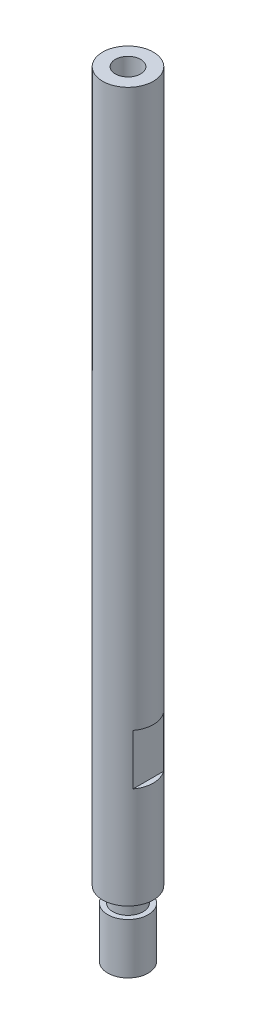
SolidWorks part; units mm, degrees
ref_plane "Front Plane" through (0, 0, 0) normal (0, 0, 1) x (1, 0, 0)
ref_plane "Top Plane" through (0, 0, 0) normal (0, 1, 0) x (1, 0, 0)
ref_plane "Right Plane" through (0, 0, 0) normal (1, 0, 0) x (0, 0, -1)
sketch "Sketch1" plane through (0, 0, 0) normal (0, 0, 1) x (1, 0, 0)
  line L0 (0, 14.171) -> (0, -138.829)
  line L1 (0, -138.829) -> (-4, -138.829)
  line L2 (-4, -138.829) -> (-4, -128.829)
  line L3 (-4, -128.829) -> (-3, -128.829)
  line L4 (-3, -128.829) -> (-3, -125.829)
  line L5 (-3, -125.829) -> (-5, -125.829)
  line L6 (-5, -125.829) -> (-5, 14.171)
  line L7 (-5, 14.171) -> (0, 14.171)
  dimension "D1" = 5
  dimension "D2" = 140
  dimension "D3" = 3
  dimension "D4" = 153
  dimension "D5" = 4
  dimension "D6" = 3
revolve "Revolve1" add sketch "Sketch1" angle 360 about L0
cosmetic thread "Cosmetic Thread1" parameters "D2"=6.647
sketch "Sketch2" plane through (0, 0, 0) normal (0, 0, 1) x (1, 0, 0)
  line L0 (-5, 14.171) -> (-5, -125.829) construction
  line L1 (-5, -95.829) -> (-4, -95.829)
  line L2 (-5, -95.829) -> (-5, -105.829)
  line L3 (-5, -105.829) -> (-4, -105.829)
  line L4 (-4, -95.829) -> (-4, -105.829)
  line L5 (5, 14.171) -> (-5, 14.171) construction
  line L6 (0, -125.829) -> (0, -35.6063) construction
  line L7 (-3, -125.829) -> (3, -125.829) construction
  line L8 (4, -95.829) -> (4, -105.829)
  line L9 (5, -105.829) -> (4, -105.829)
  line L10 (5, -95.829) -> (5, -105.829)
  line L11 (5, -95.829) -> (4, -95.829)
  point P6 (-4.5, -95.829)
  dimension "D1" = 1
  dimension "D2" = 10
  dimension "D3" = 110
extrude "Cut-Extrude1" cut sketch "Sketch2" against normal through all both and the other way through all
hole_wizard "M6 Tapped Hole1" positions "Sketch3" profile "Sketch4" tap size "M6" standard "GB"
sketch "Sketch3" plane through (0, 14.171, 0) normal (0, 1, 0) x (1, 0, 0)
  point P0 (0, 0)
sketch "Sketch4" plane through (0, 14.171, 0) normal (1, 0, 0) x (0, 0, 1)
  line L0 (0, 0) -> (0, 13.5022)
  line L1 (0, 13.5022) -> (2.5, 12)
  line L2 (2.5, 12) -> (2.5, 0)
  line L5 (2.5, 0) -> (0, 0)
  line L10 (0, 13.5022) -> (-2.5, 12) construction
  line L11 (0, -6.35) -> (0, 107.95) construction
  dimension "螺纹孔钻头直径" = 5
  dimension "螺纹孔钻头深度" = 12
  dimension "导头角度" = 118
cosmetic thread "孔螺蚊线1" parameters "D1"=8, "D2"=6
